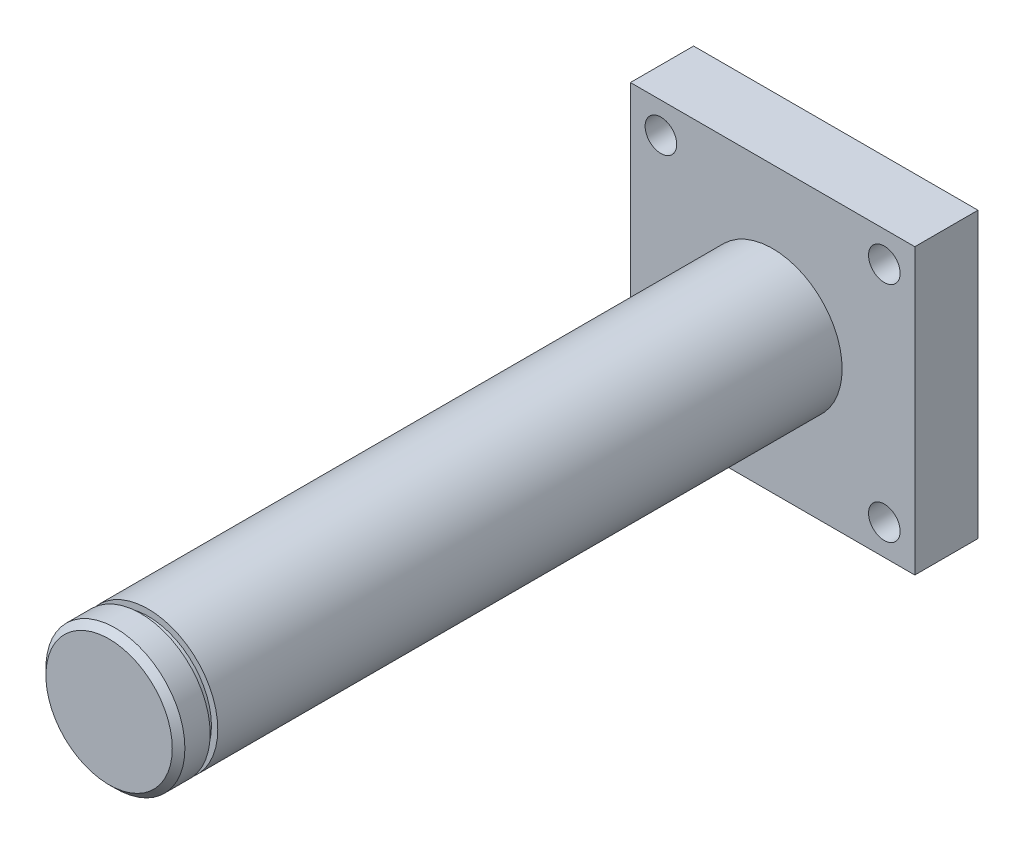
SolidWorks part; units mm, degrees
ref_plane "Front Plane" through (0, 0, 0) normal (0, 0, 1) x (1, 0, 0)
ref_plane "Top Plane" through (0, 0, 0) normal (0, 1, 0) x (1, 0, 0)
ref_plane "Right Plane" through (0, 0, 0) normal (1, 0, 0) x (0, 0, -1)
sketch "Sketch1" plane through (0, 0, 0) normal (0, 0, 1) x (1, 0, 0)
  line L1 (-22.5, 22.5) -> (22.5, 22.5)
  line L2 (-22.5, 22.5) -> (-22.5, -22.5)
  line L3 (-22.5, -22.5) -> (22.5, -22.5)
  line L4 (22.5, 22.5) -> (22.5, -22.5)
  line L5 (-22.5, 22.5) -> (22.5, -22.5) construction
  line L6 (-22.5, -22.5) -> (22.5, 22.5) construction
  circle A0 centre (0, 0) radius 25 construction
  circle A1 centre (17.6777, 17.6777) radius 2.5
  circle A2 centre (17.6777, -17.6777) radius 2.5
  circle A3 centre (-17.6777, -17.6777) radius 2.5
  circle A4 centre (-17.6777, 17.6777) radius 2.5
  point P0 (0, 0)
  point P19 (0, 0)
  dimension "D3" = 50
  dimension "D4" = 5
  dimension "D1" = 45
  dimension "D2" = 45
  dimension "D5" = 4
extrude "Boss-Extrude1" add sketch "Sketch1" along normal blind 10
sketch "Sketch2" plane through (0, 0, 10) normal (0, 0, 1) x (1, 0, 0)
  circle A0 centre (0, 0) radius 11
  dimension "D1" = 22
extrude "Boss-Extrude2" add sketch "Sketch2" along normal blind 105
chamfer "Chamfer1" distance 1 angle 45 1 edges at (11, 0, 115)
sketch "Sketch3" plane through (0, 0, 115) normal (0, 0, 1) x (1, 0, 0)
  circle A0 centre (0, 0) radius 10
  circle A1 centre (0, 0) radius 12.2484
extrude "Cut-Extrude1" cut sketch "Sketch3" against normal blind 1.2 from offset 5
